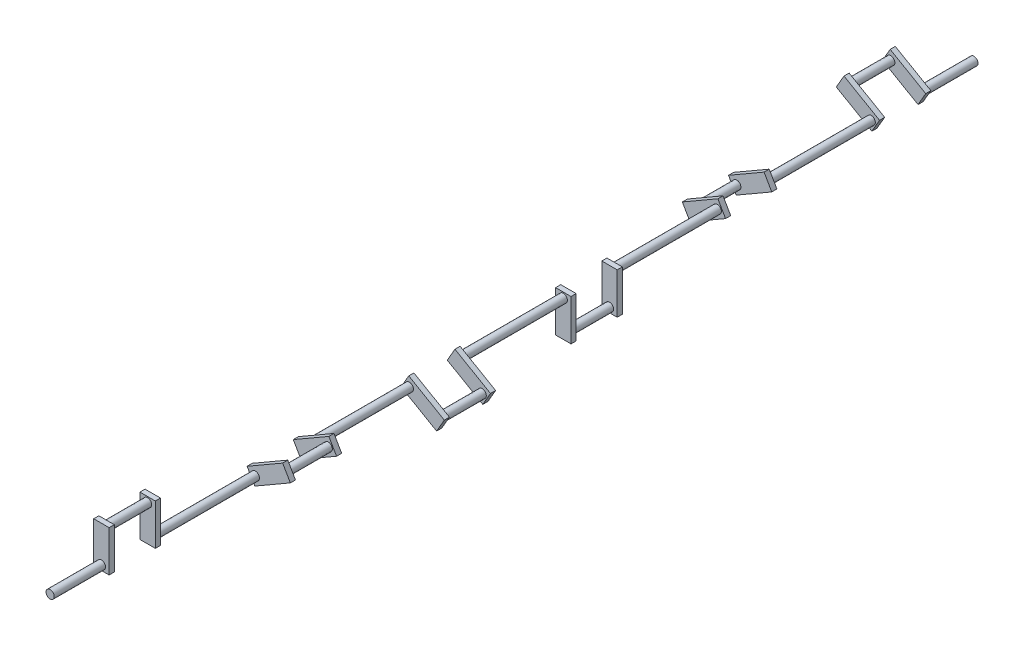
from build123d import *

# Parameters (mm, degrees)
SKETCH1_W            = 30
SKETCH1_H            = 80
SKETCH1_R            = 8
BOSS_EXTRUDE1_DEPTH  = 10
BOSS_EXTRUDE2_START  = -100
SKETCH2_R            = 8
BOSS_EXTRUDE2_DEPTH  = 100
SKETCH3_W            = 30
SKETCH3_H            = 80
SKETCH3_R            = 8
BOSS_EXTRUDE3_DEPTH  = 10
BOSS_EXTRUDE4_START  = -210
SKETCH4_R            = 8
BOSS_EXTRUDE4_DEPTH  = 210
SKETCH5_R            = 8
BOSS_EXTRUDE5_DEPTH  = 10
SKETCH6_R            = 8
BOSS_EXTRUDE6_DEPTH  = 100
BOSS_EXTRUDE7_DEPTH  = 10
BOSS_EXTRUDE8_START  = 200
SKETCH8_R            = 8
BOSS_EXTRUDE8_DEPTH  = 200
BOSS_EXTRUDE9_DEPTH  = 10
SKETCH10_R           = 8
BOSS_EXTRUDE10_DEPTH = 80
BOSS_EXTRUDE11_DEPTH = 10
BOSS_EXTRUDE12_START = 200
SKETCH12_R           = 8
BOSS_EXTRUDE12_DEPTH = 200
SKETCH13_W           = 30
SKETCH13_H           = 80
BOSS_EXTRUDE13_DEPTH = 10
SKETCH14_R           = 8
BOSS_EXTRUDE14_DEPTH = 80
SKETCH15_W           = 30
SKETCH15_H           = 80
BOSS_EXTRUDE15_DEPTH = 10
BOSS_EXTRUDE16_START = 200
SKETCH16_R           = 8
BOSS_EXTRUDE16_DEPTH = 200
BOSS_EXTRUDE17_DEPTH = 10
SKETCH18_R           = 8
BOSS_EXTRUDE18_DEPTH = 80
BOSS_EXTRUDE19_DEPTH = 10
BOSS_EXTRUDE20_START = 200
SKETCH20_R           = 8
BOSS_EXTRUDE20_DEPTH = 200
BOSS_EXTRUDE21_DEPTH = 10
SKETCH22_R           = 8
BOSS_EXTRUDE22_DEPTH = 80
BOSS_EXTRUDE23_DEPTH = 10
BOSS_EXTRUDE24_START = 100
SKETCH24_R           = 8
BOSS_EXTRUDE24_DEPTH = 100
SKETCH25_R           = 8
BOSS_EXTRUDE25_DEPTH = 110


with BuildPart() as part:
    # Sketch1 → Boss-Extrude1 (new body)
    with BuildSketch(Plane.XY):
        with Locations((15, 40)):
            Rectangle(SKETCH1_W, SKETCH1_H)
        with Locations((15, 70)):
            Circle(SKETCH1_R, mode=Mode.SUBTRACT)
        with Locations((15, 10)):
            Circle(SKETCH1_R, mode=Mode.SUBTRACT)
    extrude(amount=BOSS_EXTRUDE1_DEPTH)

    # Sketch2 → Boss-Extrude2 (add)
    with BuildSketch(Plane.XY.offset(10).offset(BOSS_EXTRUDE2_START)):
        with Locations((15, 70)):
            Circle(SKETCH2_R)
    extrude(amount=BOSS_EXTRUDE2_DEPTH)

    # Sketch3 → Boss-Extrude3 (add)
    with BuildSketch(Plane(origin=(0, 0, -90), x_dir=(-1, 0, 0), z_dir=(0, 0, -1))):
        with Locations((-15, 40)):
            Rectangle(SKETCH3_W, SKETCH3_H)
        with Locations(Location((-15, 10, 0), (0, 0, 180))):
            Circle(SKETCH3_R, mode=Mode.SUBTRACT)
    extrude(amount=-BOSS_EXTRUDE3_DEPTH)

    # Sketch4 → Boss-Extrude4 (add)
    with BuildSketch(Plane.XY.offset(-80).offset(BOSS_EXTRUDE4_START)):
        with Locations((15, 10)):
            Circle(SKETCH4_R)
    extrude(amount=BOSS_EXTRUDE4_DEPTH)

    # Sketch5 → Boss-Extrude5 (add)
    with BuildSketch(Plane(origin=(0, 0, -290), x_dir=(-1, 0, 0), z_dir=(0, 0, -1))):
        Polygon((-83.121778265, 32.009618943), (-13.839745962, -7.990381057), (1.160254038, 17.990381057), (-68.121778265, 57.990381057), align=None)
        with Locations((-66.961524227, 40)):
            Circle(SKETCH5_R, mode=Mode.SUBTRACT)
    extrude(amount=BOSS_EXTRUDE5_DEPTH)

    # Sketch6 → Boss-Extrude6 (add)
    with BuildSketch(Plane.XY.offset(-290)):
        with Locations((66.961524227, 40)):
            Circle(SKETCH6_R)
    extrude(amount=-BOSS_EXTRUDE6_DEPTH)

    # Sketch7 → Boss-Extrude7 (add)
    with BuildSketch(Plane(origin=(0, 0, -390), x_dir=(-1, 0, 0), z_dir=(0, 0, -1))):
        Polygon((-83.121778265, 32.009618943), (-13.839745962, -7.990381057), (1.160254038, 17.990381057), (-68.121778265, 57.990381057), align=None)
    extrude(amount=-BOSS_EXTRUDE7_DEPTH)

    # Sketch8 → Boss-Extrude8 (add)
    with BuildSketch(Plane(origin=(0, 0, -390), x_dir=(-1, 0, 0), z_dir=(0, 0, -1)).offset(BOSS_EXTRUDE8_START)):
        with Locations(Location((-15, 10, 0), (0, 0, 180))):
            Circle(SKETCH8_R)
    extrude(amount=-BOSS_EXTRUDE8_DEPTH)

    # Sketch9 → Boss-Extrude9 (add)
    with BuildSketch(Plane(origin=(0, 0, -590), x_dir=(-1, 0, 0), z_dir=(0, 0, -1))):
        Polygon((-68.121778265, -37.990381057), (1.160254038, 2.009618943), (-13.839745962, 27.990381057), (-83.121778265, -12.009618943), align=None)
    extrude(amount=BOSS_EXTRUDE9_DEPTH)

    # Sketch10 → Boss-Extrude10 (add)
    with BuildSketch(Plane(origin=(0, 0, -600), x_dir=(-1, 0, 0), z_dir=(0, 0, -1))):
        with Locations((-66.961524227, -20)):
            Circle(SKETCH10_R)
    extrude(amount=BOSS_EXTRUDE10_DEPTH)

    # Sketch11 → Boss-Extrude11 (add)
    with BuildSketch(Plane(origin=(0, 0, -680), x_dir=(-1, 0, 0), z_dir=(0, 0, -1))):
        Polygon((-68.121778265, -37.990381057), (-83.121778265, -12.009618943), (-13.839745962, 27.990381057), (1.160254038, 2.009618943), align=None)
    extrude(amount=BOSS_EXTRUDE11_DEPTH)

    # Sketch12 → Boss-Extrude12 (add)
    with BuildSketch(Plane(origin=(0, 0, -690), x_dir=(-1, 0, 0), z_dir=(0, 0, -1)).offset(BOSS_EXTRUDE12_START)):
        with Locations(Location((-15, 10, 0), (0, 0, 180))):
            Circle(SKETCH12_R)
    extrude(amount=-BOSS_EXTRUDE12_DEPTH)

    # Sketch13 → Boss-Extrude13 (add)
    with BuildSketch(Plane(origin=(0, 0, -890), x_dir=(-1, 0, 0), z_dir=(0, 0, -1))):
        with Locations((-15, -20)):
            Rectangle(SKETCH13_W, SKETCH13_H)
    extrude(amount=BOSS_EXTRUDE13_DEPTH)

    # Sketch14 → Boss-Extrude14 (add)
    with BuildSketch(Plane(origin=(0, 0, -900), x_dir=(-1, 0, 0), z_dir=(0, 0, -1))):
        with Locations((-15, -50)):
            Circle(SKETCH14_R)
    extrude(amount=BOSS_EXTRUDE14_DEPTH)

    # Sketch15 → Boss-Extrude15 (add)
    with BuildSketch(Plane(origin=(0, 0, -980), x_dir=(-1, 0, 0), z_dir=(0, 0, -1))):
        with Locations((-15, -20)):
            Rectangle(SKETCH15_W, SKETCH15_H)
    extrude(amount=BOSS_EXTRUDE15_DEPTH)

    # Sketch16 → Boss-Extrude16 (add)
    with BuildSketch(Plane(origin=(0, 0, -990), x_dir=(-1, 0, 0), z_dir=(0, 0, -1)).offset(BOSS_EXTRUDE16_START)):
        with Locations(Location((-15, 10, 0), (0, 0, 180))):
            Circle(SKETCH16_R)
    extrude(amount=-BOSS_EXTRUDE16_DEPTH)

    # Sketch17 → Boss-Extrude17 (add)
    with BuildSketch(Plane(origin=(0, 0, -1190), x_dir=(-1, 0, 0), z_dir=(0, 0, -1))):
        Polygon((53.121778265, -12.009618943), (-16.160254038, 27.990381057), (-31.160254038, 2.009618943), (38.121778265, -37.990381057), align=None)
    extrude(amount=BOSS_EXTRUDE17_DEPTH)

    # Sketch18 → Boss-Extrude18 (add)
    with BuildSketch(Plane(origin=(0, 0, -1200), x_dir=(-1, 0, 0), z_dir=(0, 0, -1))):
        with Locations((36.961524227, -20)):
            Circle(SKETCH18_R)
    extrude(amount=BOSS_EXTRUDE18_DEPTH)

    # Sketch19 → Boss-Extrude19 (add)
    with BuildSketch(Plane(origin=(0, 0, -1280), x_dir=(-1, 0, 0), z_dir=(0, 0, -1))):
        Polygon((53.121778265, -12.009618943), (38.121778265, -37.990381057), (-31.160254038, 2.009618943), (-16.160254038, 27.990381057), align=None)
    extrude(amount=BOSS_EXTRUDE19_DEPTH)

    # Sketch20 → Boss-Extrude20 (add)
    with BuildSketch(Plane(origin=(0, 0, -1290), x_dir=(-1, 0, 0), z_dir=(0, 0, -1)).offset(BOSS_EXTRUDE20_START)):
        with Locations(Location((-15, 10, 0), (0, 0, 180))):
            Circle(SKETCH20_R)
    extrude(amount=-BOSS_EXTRUDE20_DEPTH)

    # Sketch21 → Boss-Extrude21 (add)
    with BuildSketch(Plane(origin=(0, 0, -1490), x_dir=(-1, 0, 0), z_dir=(0, 0, -1))):
        Polygon((38.121778265, 57.990381057), (-31.160254038, 17.990381057), (-16.160254038, -7.990381057), (53.121778265, 32.009618943), align=None)
    extrude(amount=BOSS_EXTRUDE21_DEPTH)

    # Sketch22 → Boss-Extrude22 (add)
    with BuildSketch(Plane(origin=(0, 0, -1500), x_dir=(-1, 0, 0), z_dir=(0, 0, -1))):
        with Locations((36.961524227, 40)):
            Circle(SKETCH22_R)
    extrude(amount=BOSS_EXTRUDE22_DEPTH)

    # Sketch23 → Boss-Extrude23 (add)
    with BuildSketch(Plane(origin=(0, 0, -1580), x_dir=(-1, 0, 0), z_dir=(0, 0, -1))):
        Polygon((38.121778265, 57.990381057), (53.121778265, 32.009618943), (-16.160254038, -7.990381057), (-31.160254038, 17.990381057), align=None)
    extrude(amount=BOSS_EXTRUDE23_DEPTH)

    # Sketch24 → Boss-Extrude24 (add)
    with BuildSketch(Plane(origin=(0, 0, -1590), x_dir=(-1, 0, 0), z_dir=(0, 0, -1)).offset(BOSS_EXTRUDE24_START)):
        with Locations(Location((-15, 10, 0), (0, 0, 180))):
            Circle(SKETCH24_R)
    extrude(amount=-BOSS_EXTRUDE24_DEPTH)

    # Sketch25 → Boss-Extrude25 (add)
    with BuildSketch(Plane(origin=(0, 0, 0), x_dir=(-1, 0, 0), z_dir=(0, 0, -1))):
        with Locations(Location((-15, 10, 0), (0, 0, 180))):
            Circle(SKETCH25_R)
    extrude(amount=-BOSS_EXTRUDE25_DEPTH)


solid = part.part
